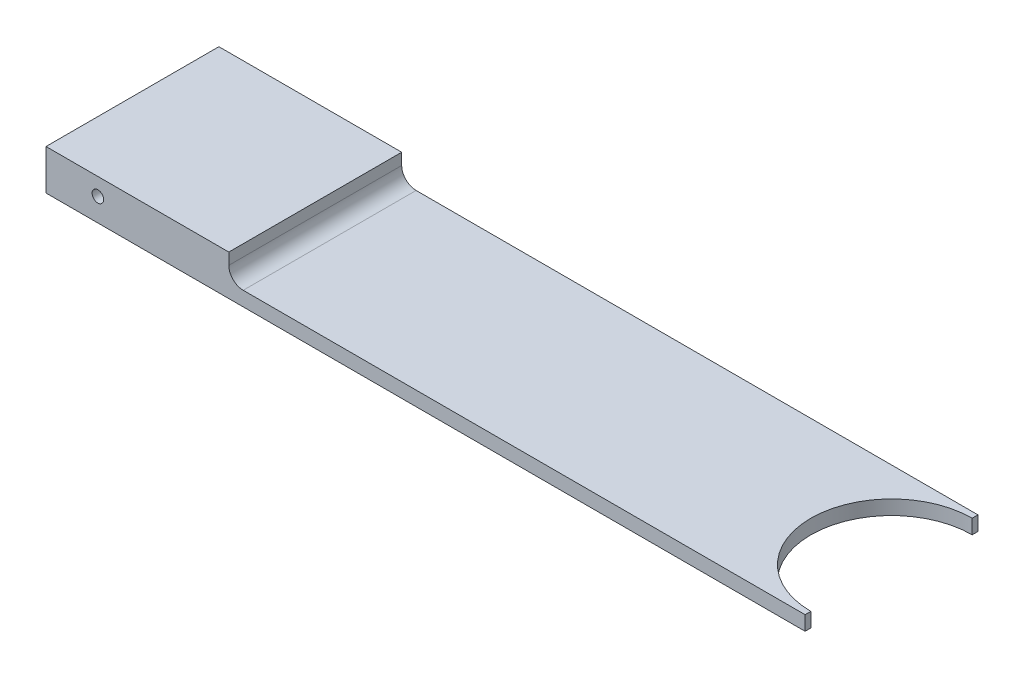
SolidWorks part; units mm, degrees
ref_plane "Front Plane" through (0, 0, 0) normal (0, 0, 1) x (1, 0, 0)
ref_plane "Top Plane" through (0, 0, 0) normal (0, 1, 0) x (1, 0, 0)
ref_plane "Right Plane" through (0, 0, 0) normal (1, 0, 0) x (0, 0, -1)
sketch "Sketch2" plane through (0, 0, 0) normal (0, 1, 0) x (1, 0, 0)
  line L1 (-50, 30) -> (50, 30)
  line L2 (-50, 30) -> (-50, -30)
  line L3 (-50, -30) -> (50, -30)
  line L5 (-50, 30) -> (50, -30) construction
  line L6 (-50, -30) -> (50, 30) construction
  line L7 (0, 0) -> (57.8907, 0) construction
  line L8 (50, -38.0505) -> (50, 37.5717) construction
  line L10 (50, -30) -> (150, -30)
  line L11 (150, -30) -> (150, -28)
  line L12 (150, 30) -> (50, 30)
  line L13 (150, 28) -> (150, 30)
  arc A0 (150, 28) -> (150, -28) centre (150, 0) ccw
  point P0 (0, 0)
  dimension "D3" = 100
  dimension "D4" = 56
  dimension "D1" = 60
  dimension "D2" = 100
extrude "Boss-Extrude2" add sketch "Sketch2" along normal mid plane 5
sketch "Sketch5" plane through (0, 0, 0) normal (0, 0, 1) x (1, 0, 0)
  line L1 (-50, -2.5) -> (-113.4393, -2.5)
  line L2 (-50, -2.5) -> (-50, 11.4912)
  line L3 (-50, 11.4912) -> (-113.4393, 11.4912)
  line L4 (-113.4393, -2.5) -> (-113.4393, 11.4912)
  dimension "D1" = 63.4393
extrude "Boss-Extrude3" add sketch "Sketch5" along normal mid plane 60
fillet "Fillet1" radius 5 1 edges
sketch "Sketch6" plane through (0, 0, 30) normal (0, 0, 1) x (1, 0, 0)
  line L0 (-95.4393, 26.929) -> (-95.4393, -14.1765) construction
  line L1 (-125.6234, 5.4912) -> (-65.2436, 5.4912) construction
  line L2 (-50, 11.4912) -> (-113.4393, 11.4912) construction
  line L3 (-113.4393, 11.4912) -> (-113.4393, -2.5) construction
  circle A0 centre (-95.4393, 5.4912) radius 2
  dimension "D1" = 4
  dimension "D2" = 6
  dimension "D3" = 18
extrude "Cut-Extrude1" cut sketch "Sketch6" against normal through all
